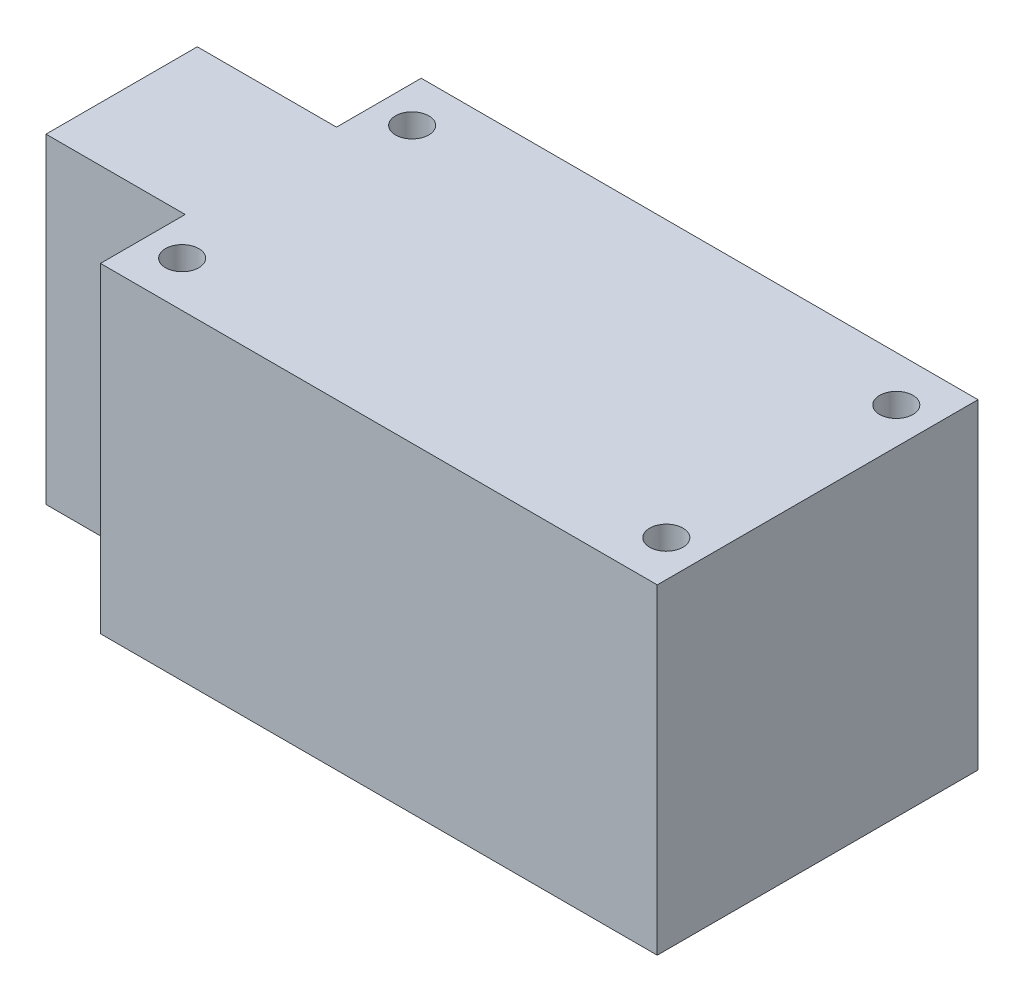
from build123d import *

# Parameters (mm, degrees)
SKETCH_1_W          = 115
SKETCH_1_H          = 53
EXTRUDE_1_DEPTH     = 53
SKETCH_2_W          = 46
SKETCH_2_H          = 28
CUT_EXTRUDE_1_DEPTH = 83.568153667
SKETCH_3_R          = 2.75
CUT_EXTRUDE_2_DEPTH = 83.568153667


with BuildPart() as part:
    # 草图1 → 凸台-拉伸1 (new body)
    with BuildSketch(Plane(origin=(0, 0, 0), x_dir=(1, 0, 0), z_dir=(0, 1, 0))):
        Rectangle(SKETCH_1_W, SKETCH_1_H)
    extrude(amount=EXTRUDE_1_DEPTH)

    # 草图2 → 切除-拉伸1 (cut, through all)
    with BuildSketch(Plane(origin=(0, 53, 0), x_dir=(1, 0, 0), z_dir=(0, 1, 0))):
        with Locations((-57.5, -26.5)):
            Rectangle(SKETCH_2_W, SKETCH_2_H)
        with Locations((-57.5, 26.5)):
            Rectangle(SKETCH_2_W, SKETCH_2_H)
    extrude(amount=-CUT_EXTRUDE_1_DEPTH, mode=Mode.SUBTRACT)

    # 草图3 → 切除-拉伸2 (cut, through all)
    with BuildSketch(Plane(origin=(0, 53, 0), x_dir=(1, 0, 0), z_dir=(0, 1, 0))):
        with Locations(Location((-28.5, 19, 0), (0, 0, 270))):
            Circle(SKETCH_3_R)
        with Locations(Location((51.5, 19, 0), (0, 0, 270))):
            Circle(SKETCH_3_R)
        with Locations(Location((51.5, -19, 0), (0, 0, 270))):
            Circle(SKETCH_3_R)
        with Locations(Location((-28.5, -19, 0), (0, 0, 270))):
            Circle(SKETCH_3_R)
    extrude(amount=-CUT_EXTRUDE_2_DEPTH, mode=Mode.SUBTRACT)


solid = part.part
